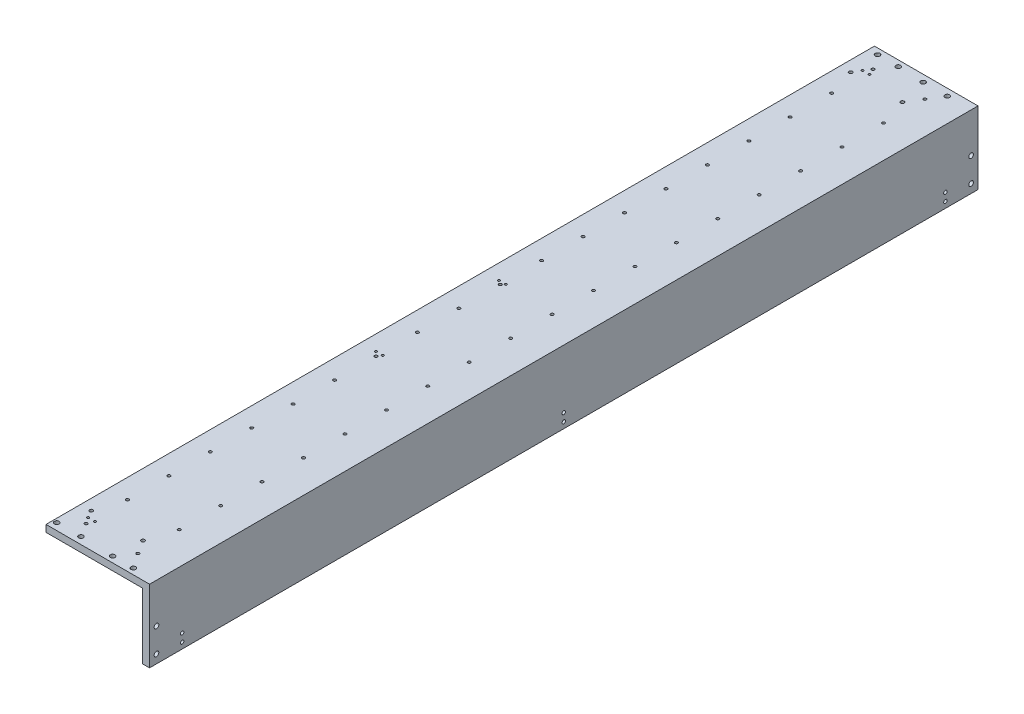
SolidWorks part; units mm, degrees
material "6061Al"
ref_plane "前视基准面" through (0, 0, 0) normal (0, 0, 1) x (1, 0, 0)
ref_plane "上视基准面" through (0, 0, 0) normal (0, 1, 0) x (1, 0, 0)
ref_plane "右视基准面" through (0, 0, 0) normal (1, 0, 0) x (0, 0, -1)
sketch "草图1" plane through (0, 0, 0) normal (0, 0, 1) x (1, 0, 0)
  line L0 (0, 0) -> (160, 0)
  line L1 (160, 0) -> (160, -105)
  line L2 (0, -10) -> (150, -10)
  line L3 (150, -10) -> (150, -105)
  line L4 (0, 0) -> (0, -10)
  line L5 (150, -105) -> (160, -105)
  dimension "D1" = 160
  dimension "D2" = 105
  dimension "D3" = 10
extrude "凸台-拉伸1" add sketch "草图1" along normal mid plane 1200
hole_wizard "M8 螺纹孔1" positions "草图3" profile "草图4" tap size "M8" standard "ISO" end condition through all
sketch "草图3" plane through (0, 0, 0) normal (0, 1, 0) x (1, 0, 0)
  line L0 (0, 0) -> (239.8955, 0) construction
  point P0 (15.5, -590)
  point P3 (50.5, -590)
  point P14 (90.5, 590)
  point P17 (125.5, 590)
sketch "草图4" plane through (15.5, 0, 590) normal (1, 0, 0) x (0, 0, 1)
  line L0 (0, 0) -> (0, 105)
  line L1 (0, 105) -> (3.4, 105)
  line L2 (3.4, 105) -> (3.4, 0)
  line L5 (3.4, 0) -> (0, 0)
  line L11 (0, -6.35) -> (0, 107.95) construction
  dimension "通孔螺纹孔钻头直径" = 6.8
  dimension "通孔螺纹孔钻头深度" = 105
cosmetic thread "孔螺蚊线1"
cosmetic thread "孔螺蚊线2"
cosmetic thread "孔螺蚊线47"
cosmetic thread "孔螺蚊线48"
hole_wizard "M8 螺纹孔2" positions "草图5" profile "草图6" tap size "M8" standard "ISO" end condition through all
sketch "草图5" plane through (160, 0, 0) normal (1, 0, 0) x (0, 0, -1)
  line L0 (0, 0) -> (0, -165.87) construction
  point P0 (-590, -57.5)
  point P3 (-590, -92.5)
  point P12 (590, -92.5)
  point P13 (590, -57.5)
sketch "草图6" plane through (160, -57.5, 590) normal (0, 1, 0) x (0, 0, -1)
  line L0 (0, 0) -> (0, 160)
  line L1 (0, 160) -> (3.4, 160)
  line L2 (3.4, 160) -> (3.4, 0)
  line L5 (3.4, 0) -> (0, 0)
  line L11 (0, -6.35) -> (0, 107.95) construction
  dimension "通孔螺纹孔钻头直径" = 6.8
  dimension "通孔螺纹孔钻头深度" = 160
cosmetic thread "孔螺蚊线23"
cosmetic thread "孔螺蚊线24"
cosmetic thread "孔螺蚊线45"
cosmetic thread "孔螺蚊线46"
hole_wizard "M5 螺纹孔1" positions "草图7" profile "草图8" tap size "M5" standard "ISO" end condition through all
sketch "草图7" plane through (0, -10, 0) normal (0, -1, 0) x (-1, 0, 0)
  line L0 (-38, -570) -> (-38, -510) construction
  line L1 (-113, -570) -> (-113, -510) construction
  line L2 (-38, 570) -> (-113, 570) construction
  point P0 (-38, -570)
  point P8 (-38, -510)
  point P9 (-38, -450)
  point P10 (-38, -390)
  point P11 (-38, -330)
  point P12 (-38, -270)
  point P13 (-38, -210)
  point P14 (-38, -150)
  point P15 (-38, -90)
  point P16 (-38, -30)
  point P17 (-38, 30)
  point P18 (-38, 90)
  point P19 (-38, 150)
  point P20 (-38, 210)
  point P21 (-38, 270)
  point P22 (-38, 330)
  point P23 (-38, 390)
  point P24 (-38, 450)
  point P25 (-38, 510)
  point P26 (-38, 570)
  point P31 (-113, -570)
  point P32 (-113, -510)
  point P33 (-113, -450)
  point P34 (-113, -390)
  point P35 (-113, -330)
  point P36 (-113, -270)
  point P37 (-113, -210)
  point P38 (-113, -150)
  point P39 (-113, -90)
  point P40 (-113, -30)
  point P41 (-113, 30)
  point P42 (-113, 90)
  point P43 (-113, 150)
  point P44 (-113, 210)
  point P45 (-113, 270)
  point P46 (-113, 330)
  point P47 (-113, 390)
  point P48 (-113, 450)
  point P49 (-113, 510)
  point P50 (-113, 570)
  dimension "D2" = 60
  dimension "D4" = 75
  dimension "D1" = 20
  dimension "D3" = 2
sketch "草图8" plane through (38, -10, 570) normal (1, 0, 0) x (0, 0, -1)
  line L0 (0, 0) -> (0, 10)
  line L1 (0, 10) -> (2.1, 10)
  line L2 (2.1, 10) -> (2.1, 0)
  line L5 (2.1, 0) -> (0, 0)
  line L11 (0, -6.35) -> (0, 107.95) construction
  dimension "通孔螺纹孔钻头直径" = 4.2
  dimension "通孔螺纹孔钻头深度" = 10
cosmetic thread "孔螺蚊线3"
cosmetic thread "孔螺蚊线4"
cosmetic thread "孔螺蚊线5"
cosmetic thread "孔螺蚊线6"
cosmetic thread "孔螺蚊线7"
cosmetic thread "孔螺蚊线8"
cosmetic thread "孔螺蚊线9"
cosmetic thread "孔螺蚊线10"
cosmetic thread "孔螺蚊线11"
cosmetic thread "孔螺蚊线12"
cosmetic thread "孔螺蚊线13"
cosmetic thread "孔螺蚊线14"
cosmetic thread "孔螺蚊线15"
cosmetic thread "孔螺蚊线16"
cosmetic thread "孔螺蚊线17"
cosmetic thread "孔螺蚊线18"
cosmetic thread "孔螺蚊线19"
cosmetic thread "孔螺蚊线20"
cosmetic thread "孔螺蚊线21"
cosmetic thread "孔螺蚊线22"
cosmetic thread "孔螺蚊线25"
cosmetic thread "孔螺蚊线26"
cosmetic thread "孔螺蚊线27"
cosmetic thread "孔螺蚊线28"
cosmetic thread "孔螺蚊线29"
cosmetic thread "孔螺蚊线30"
cosmetic thread "孔螺蚊线31"
cosmetic thread "孔螺蚊线32"
cosmetic thread "孔螺蚊线33"
cosmetic thread "孔螺蚊线34"
cosmetic thread "孔螺蚊线35"
cosmetic thread "孔螺蚊线36"
cosmetic thread "孔螺蚊线37"
cosmetic thread "孔螺蚊线38"
cosmetic thread "孔螺蚊线39"
cosmetic thread "孔螺蚊线40"
cosmetic thread "孔螺蚊线41"
cosmetic thread "孔螺蚊线42"
cosmetic thread "孔螺蚊线43"
cosmetic thread "孔螺蚊线44"
hole_wizard "Ø5.0mm 暗销孔1" positions "草图9" profile "草图10" hole size "Ø5.0" standard "ISO" end condition through all
sketch "草图9" plane through (0, -10, 0) normal (0, -1, 0) x (-1, 0, 0)
  line L0 (-28, 600) -> (-28, 157.6) construction
  line L1 (0, 600) -> (-150, 600) construction
  line L2 (0, 0) -> (303.823, 0) construction
  line L3 (-25.5, -550) -> (-100.5, -550) construction
  point P0 (-25.5, 550)
  point P11 (-25.5, -550)
  point P14 (-100.5, 550)
  point P15 (-100.5, -550)
  dimension "D1" = 2.5
  dimension "D2" = 50
  dimension "D3" = 2
  dimension "D4" = 75
sketch "草图10" plane through (25.5, -10, -550) normal (1, 0, 0) x (0, 0, -1)
  line L0 (0, 0) -> (0, 10)
  line L1 (0, 10) -> (2.5, 10)
  line L2 (2.5, 10) -> (2.5, 0)
  line L5 (2.5, 0) -> (0, 0)
  line L11 (0, -6.35) -> (0, 107.95) construction
  dimension "通孔孔直径" = 5
  dimension "通孔孔深度" = 10
hole_wizard "M4 螺纹孔1" positions "草图11" profile "草图12" tap size "M4" standard "ISO" end condition through all
sketch "草图11" plane through (0, 0, 0) normal (0, 1, 0) x (1, 0, 0)
  point P0 (31.9782, 560.9)
  point P3 (41.8782, 560.9)
  point P6 (31.9782, 34.1)
  point P9 (41.8782, 34.1)
  point P12 (31.9782, -144.1)
  point P15 (41.8782, -144.1)
  point P18 (31.9782, -560.9)
  point P21 (41.8782, -560.9)
sketch "草图12" plane through (31.9782, 0, -560.9) normal (1, 0, 0) x (0, 0, 1)
  line L0 (0, 0) -> (0, 105)
  line L1 (0, 105) -> (1.65, 105)
  line L2 (1.65, 105) -> (1.65, 0)
  line L5 (1.65, 0) -> (0, 0)
  line L11 (0, -6.35) -> (0, 107.95) construction
  dimension "通孔螺纹孔钻头直径" = 3.3
  dimension "通孔螺纹孔钻头深度" = 105
cosmetic thread "孔螺蚊线49"
cosmetic thread "孔螺蚊线50"
cosmetic thread "孔螺蚊线51"
cosmetic thread "孔螺蚊线52"
cosmetic thread "孔螺蚊线53"
cosmetic thread "孔螺蚊线54"
cosmetic thread "孔螺蚊线55"
cosmetic thread "孔螺蚊线56"
hole_wizard "M6 螺纹孔1" positions "草图13" profile "草图14" tap size "M6" standard "ISO" end condition through all
sketch "草图13" plane through (160, 0, 0) normal (1, 0, 0) x (0, 0, -1)
  point P0 (-552.8, -84.791)
  point P3 (-552.8, -96.291)
  point P6 (0, -84.791)
  point P9 (0, -96.291)
  point P12 (552.8, -84.791)
  point P15 (552.8, -96.291)
sketch "草图14" plane through (160, -84.791, 552.8) normal (0, 1, 0) x (0, 0, -1)
  line L0 (0, 0) -> (0, 160)
  line L1 (0, 160) -> (2.5, 160)
  line L2 (2.5, 160) -> (2.5, 0)
  line L5 (2.5, 0) -> (0, 0)
  line L11 (0, -6.35) -> (0, 107.95) construction
  dimension "通孔螺纹孔钻头直径" = 5
  dimension "通孔螺纹孔钻头深度" = 160
cosmetic thread "孔螺蚊线57"
cosmetic thread "孔螺蚊线58"
cosmetic thread "孔螺蚊线59"
cosmetic thread "孔螺蚊线60"
cosmetic thread "孔螺蚊线61"
cosmetic thread "孔螺蚊线62"
other "移动面1" face at (0, -5, 0) parameters "D1"=10
hole_wizard "M8 螺纹孔3" positions "草图15" profile "草图16" tap size "M8" standard "ISO" end condition through all
sketch "草图15" plane through (0, -10, 0) normal (0, -1, 0) x (-1, 0, 0)
  line L4 (-10, -600) -> (-150, -600) construction
  line L5 (-10, 600) -> (-150, 600) construction
  line L6 (-38, 570) -> (-38, 629.0287) construction
  line L7 (-113, -570) -> (-113, -619.7092) construction
  point P0 (-53, 591.5)
  point P2 (-23, 591.5)
  point P4 (-128, -591.5)
  point P6 (-98, -591.5)
  dimension "D1" = 30
  dimension "D2" = 8.5
  dimension "D3" = 8.5
  dimension "D4" = 30
sketch "草图16" plane through (53, -10, -591.5) normal (1, 0, 0) x (0, 0, -1)
  line L0 (0, 0) -> (0, 10)
  line L1 (0, 10) -> (3.4, 10)
  line L2 (3.4, 10) -> (3.4, 0)
  line L5 (3.4, 0) -> (0, 0)
  line L11 (0, -6.35) -> (0, 107.95) construction
  dimension "通孔螺纹孔钻头直径" = 6.8
  dimension "通孔螺纹孔钻头深度" = 10
cosmetic thread "孔螺蚊线63"
cosmetic thread "孔螺蚊线64"
cosmetic thread "孔螺蚊线65"
cosmetic thread "孔螺蚊线66"
